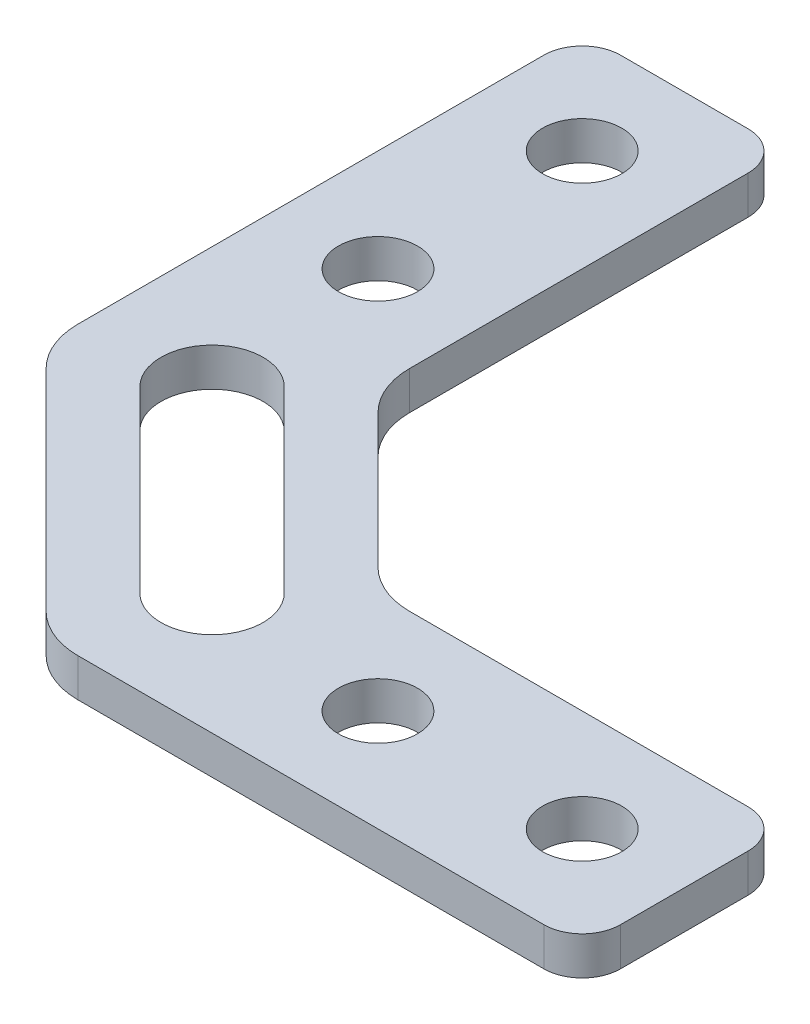
SolidWorks part; units mm, degrees
material "Thornel Mat VMA"
ref_plane "前视基准面" through (0, 0, 0) normal (0, 0, 1) x (1, 0, 0)
ref_plane "上视基准面" through (0, 0, 0) normal (0, 1, 0) x (1, 0, 0)
ref_plane "右视基准面" through (0, 0, 0) normal (1, 0, 0) x (0, 0, -1)
other "Configuration Table"
sketch "草图1" plane through (0, 0, 0) normal (0, 1, 0) x (1, 0, 0)
  line L0 (0, 0) -> (146.1035, 0) construction
  line L1 (0, 0) -> (0, 97.848) construction
  line L2 (0, 0) -> (93.9341, 93.9341) construction
  line L7 (11, 4) -> (80.0939, 4) construction
  line L9 (11, 4) -> (11, -4) construction
  line L10 (11, -4) -> (60.894, -4) construction
  line L11 (-4, 68.504) -> (-4, 11) construction
  line L12 (-4, 11) -> (4, 11) construction
  line L13 (4, 11) -> (4, 65.5955) construction
  line L14 (27, -4) -> (27, 4)
  line L15 (27, -4) -> (6, -4)
  line L16 (6, -4) -> (-4, 6)
  line L17 (27, 4) -> (11, 4)
  line L18 (11, 4) -> (4, 11)
  line L19 (-4, 27) -> (-4, 6)
  line L20 (-4, 27) -> (4, 27)
  line L21 (4, 27) -> (4, 11)
  line L22 (0.75, 7.75) -> (7.75, 0.75) construction
  line L23 (2.1642, 9.1642) -> (9.1642, 2.1642)
  line L24 (-0.6642, 6.3358) -> (6.3358, -0.6642)
  circle A0 centre (15, 0) radius 1.55
  circle A1 centre (23, 0) radius 1.55
  circle A2 centre (0, 23) radius 1.55
  circle A3 centre (0, 15) radius 1.55
  arc A4 (2.1642, 9.1642) -> (-0.6642, 6.3358) centre (0.75, 7.75) ccw
  arc A5 (6.3358, -0.6642) -> (9.1642, 2.1642) centre (7.75, 0.75) ccw
  point P25 (4.25, 4.25)
  point P27 (1, 1)
  point P34 (7.5, 7.5)
  dimension "D5" = 3.1
  dimension "D6" = 4
  dimension "D7" = 8
  dimension "D8" = 4
  dimension "D12" = 2
  dimension "D1" = 45
  dimension "D2" = 8
  dimension "D3" = 15
  dimension "D4" = 15
  dimension "D9" = 10
  dimension "D10" = 15
  dimension "D11" = 7
extrude "凸台-拉伸1" add sketch "草图1" along normal blind 1.5
fillet "圆角1" radius 1.5 4 edges at (27, 0.75, 4) (27, 0.75, -4) (4, 0.75, -27) (-4, 0.75, -27)
fillet "圆角2" radius 3 4 edges at (4, 0.75, -11) (11, 0.75, -4) (6, 0.75, 4) (-4, 0.75, -6)
